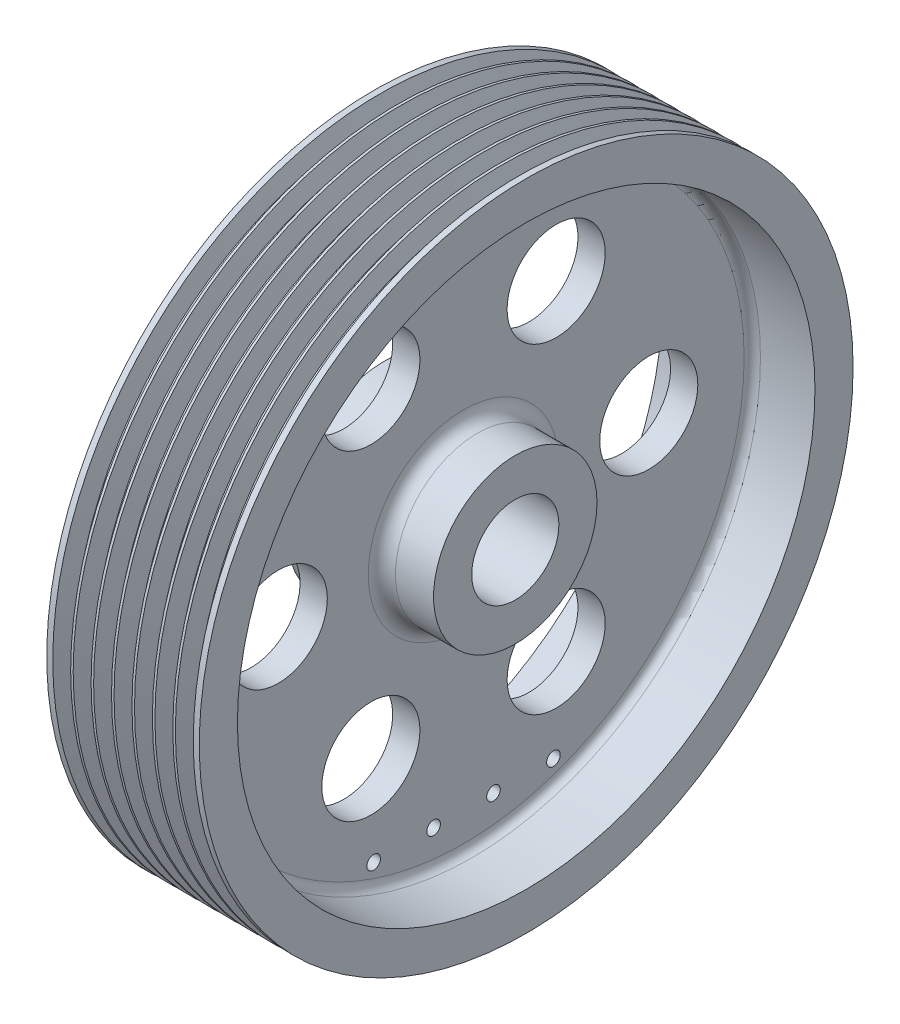
from build123d import *

# Parameters (mm, degrees)
SKETCH4_R          = 90
CUT_EXTRUDE1_DEPTH = 343
CIRPATTERN1_COUNT  = 6
CIRPATTERN2_COUNT  = 3
SKETCH8_R          = 12.5
CUT_EXTRUDE3_DEPTH = 238
LPATTERN1_COUNT    = 7
LPATTERN1_PITCH    = 37.5


with BuildPart() as part:
    # Sketch2 → Revolve1 (revolve)
    with BuildSketch(Plane.XY, mode=Mode.PRIVATE) as revolve1_sk:
        with BuildLine():
            Line((-20, 600), (-20, 530))
            Line((-20, 530), (80, 530))
            ThreePointArc((80, 530), (90.606601718, 525.606601718), (95, 515))
            Line((95, 515), (95, 205))
            ThreePointArc((95, 205), (87.67766953, 187.32233047), (70, 180))
            Line((70, 180), (0, 180))
            Line((0, 180), (0, 105))
            Line((0, 105), (70, 105))
            Line((70, 105), (70, 80))
            Line((70, 80), (240, 80))
            Line((240, 80), (240, 150))
            Line((240, 150), (170, 150))
            ThreePointArc((170, 150), (152.32233047, 157.32233047), (145, 175))
            Line((145, 175), (145, 515))
            ThreePointArc((145, 515), (149.393398282, 525.606601718), (160, 530))
            Line((160, 530), (260, 530))
            Line((260, 530), (260, 600))
            Line((260, 600), (-20, 600))
        make_face()
    revolve(revolve1_sk.sketch.rotate(Axis((225.657059372, 0, 0), (-1, 0, 0)), 90), axis=Axis((225.657059372, 0, 0), (-1, 0, 0)))

    # Sketch4 → Cut-Extrude1 (cut)
    with BuildSketch(Plane(origin=(0, 0, 0), x_dir=(0, 0, -1), z_dir=(1, 0, 0))):
        with Locations(Location((-170, 294.448637287, 0), (0, 0, 180))):
            Circle(SKETCH4_R)
    cut_extrude1 = extrude(amount=CUT_EXTRUDE1_DEPTH, mode=Mode.SUBTRACT)

    # CirPattern1: Cut-Extrude1 ×6 about axis
    cirpattern1_axis = Axis((0, 0, 0), (1, 0, 0))
    for i in range(1, CIRPATTERN1_COUNT):
        add(cut_extrude1.rotate(cirpattern1_axis, i * 360 / CIRPATTERN1_COUNT), mode=Mode.SUBTRACT)

    # Sketch6 → M24 Tapped Hole1 (revolve, cut)
    with BuildSketch(Plane(origin=(0, 114.748366001, 66.25), x_dir=(0, 0, 1), z_dir=(0, 1, 0))):
        Polygon((0, 0), (0, 46.3090365), (10.5, 40), (10.5, 0), align=None)
    m24_tapped_hole1 = revolve(axis=Axis((-6.35, 114.748366001, 66.25), (1, 0, 0)), mode=Mode.SUBTRACT)

    # CirPattern2: M24 Tapped Hole1 ×3 about axis
    cirpattern2_axis = Axis((0, 0, 0), (1, 0, 0))
    for i in range(1, CIRPATTERN2_COUNT):
        add(m24_tapped_hole1.rotate(cirpattern2_axis, i * 360 / CIRPATTERN2_COUNT), mode=Mode.SUBTRACT)

    # Sketch8 → Cut-Extrude3 (cut)
    with BuildSketch(Plane(origin=(0, 0, 0), x_dir=(0, 0, -1), z_dir=(1, 0, 0))):
        with Locations(Location((-55, -462, 0), (0, 0, 180))):
            Circle(SKETCH8_R)
        with Locations(Location((-165, -462, 0), (0, 0, 180))):
            Circle(SKETCH8_R)
        with Locations(Location((55, -462, 0), (0, 0, 180))):
            Circle(SKETCH8_R)
        with Locations(Location((165, -462, 0), (0, 0, 180))):
            Circle(SKETCH8_R)
    extrude(amount=CUT_EXTRUDE3_DEPTH, mode=Mode.SUBTRACT)

    # Sketch9 → Cut-Revolve1 (revolve, cut)
    with BuildSketch(Plane.XY, mode=Mode.PRIVATE) as cut_revolve1_sk:
        Polygon((-8.926784713, 600), (0.886552266, 571.5), (14.113447734, 571.5), (23.926784713, 600), align=None)
    cut_revolve1 = revolve(cut_revolve1_sk.sketch.rotate(Axis((0, 0, 0), (1, 0, 0)), 90), axis=Axis((0, 0, 0), (1, 0, 0)), mode=Mode.SUBTRACT)

    # LPattern1: Cut-Revolve1 ×7
    with Locations(*[(i * LPATTERN1_PITCH, 0, 0) for i in range(1, LPATTERN1_COUNT)]):
        add(cut_revolve1, mode=Mode.SUBTRACT)


solid = part.part
